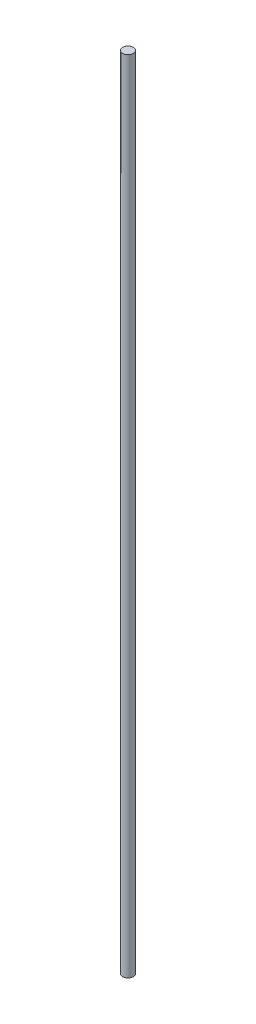
from build123d import *

# Parameters (mm, degrees)
SKETCH_1_R      = 2
EXTRUDE_1_DEPTH = 300


with BuildPart() as part:
    # 草图1 → 凸台-拉伸1 (new body)
    with BuildSketch(Plane(origin=(0, 0, 0), x_dir=(1, 0, 0), z_dir=(0, 1, 0))):
        with Locations(Location((0, 0, 0), (0, 0, 270))):
            Circle(SKETCH_1_R)
    extrude(amount=EXTRUDE_1_DEPTH)


solid = part.part
